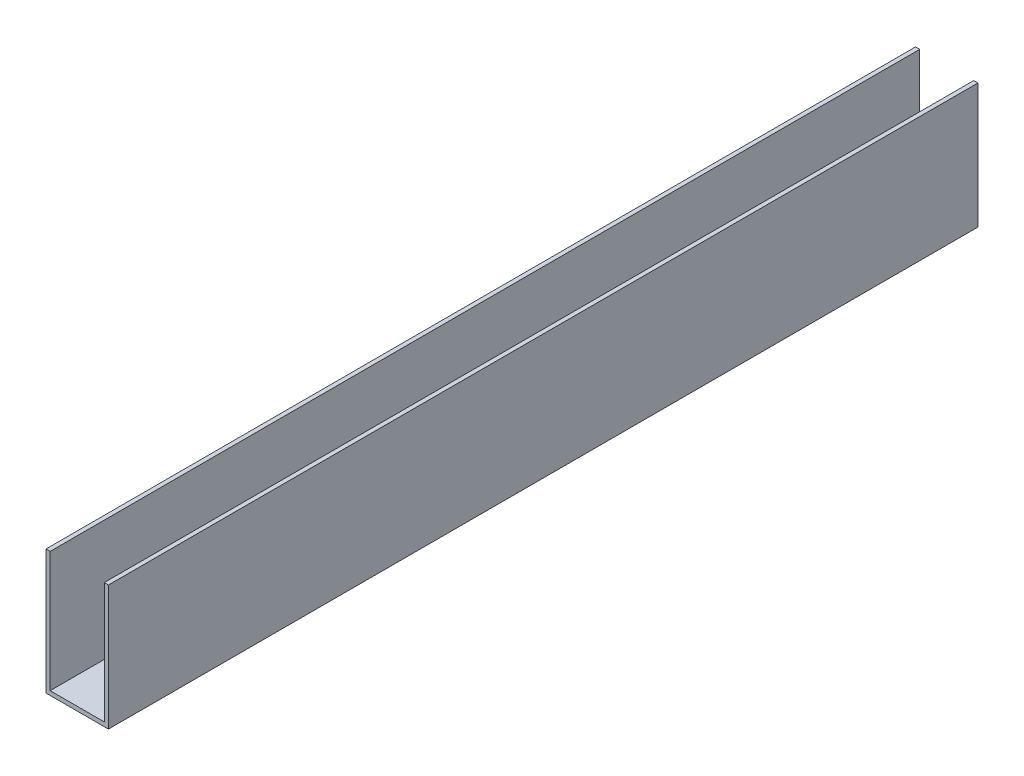
from build123d import *

# Parameters (mm, degrees)
SKETCH_1_W      = 30
SKETCH_1_H      = 60
EXTRUDE_1_DEPTH = 209
SHELL_1_T       = -2


with BuildPart() as part:
    # 草图1 → 凸台-拉伸1 (new, symmetric)
    with BuildSketch(Plane.XY):
        Rectangle(SKETCH_1_W, SKETCH_1_H)
    extrude(amount=EXTRUDE_1_DEPTH, both=True)

    # 抽壳1
    shell_1_openings = [part.faces().sort_by_distance(p)[0] for p in [
        (0, 0, 209),
        (0, 0, -209),
        (0, 30, 0),
    ]]
    offset(amount=SHELL_1_T, openings=shell_1_openings, kind=Kind.INTERSECTION)


solid = part.part
